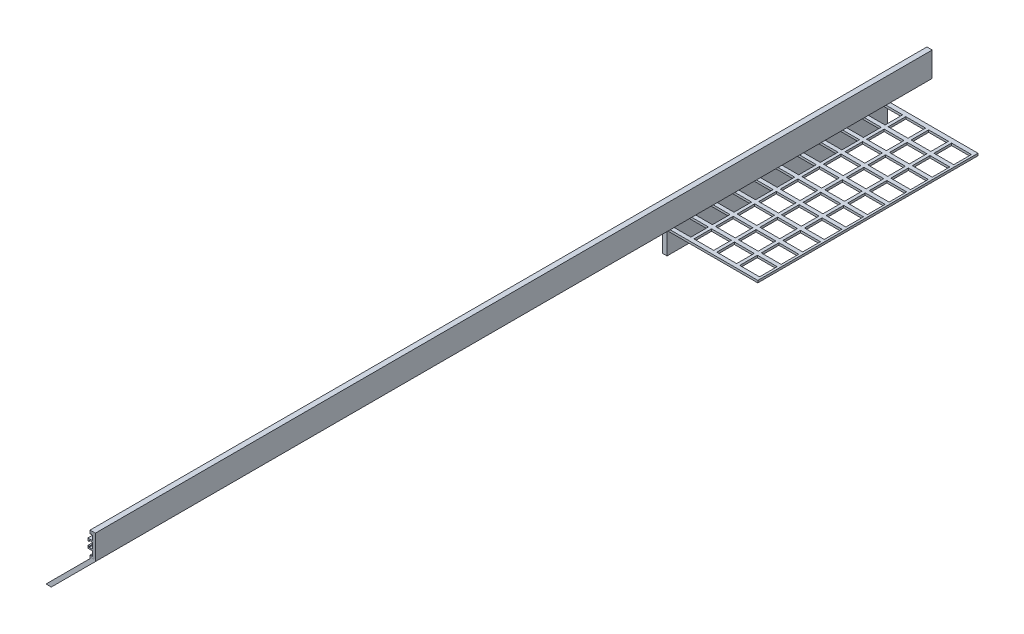
SolidWorks part; units mm, degrees
ref_plane "前视基准面" through (0, 0, 0) normal (0, 0, 1) x (1, 0, 0)
ref_plane "上视基准面" through (0, 0, 0) normal (0, 1, 0) x (1, 0, 0)
ref_plane "右视基准面" through (0, 0, 0) normal (1, 0, 0) x (0, 0, -1)
sketch "草图1" plane through (0, 0, 0) normal (0, 0, 1) x (1, 0, 0)
  line L0 (0, 0) -> (36.8328, 0) construction
  line L1 (3, -25) -> (3, 25)
  line L2 (3, 25) -> (-3, 25)
  line L3 (-3, 25) -> (-3, 21)
  line L4 (-3, 21) -> (0, 21)
  line L5 (0, 21) -> (0, 10)
  line L6 (0, 10) -> (-11, 10)
  line L7 (-11, 10) -> (-11, 4.6)
  line L8 (-11, 4.6) -> (-8, 4.6)
  line L9 (-8, 4.6) -> (-8, 7)
  line L10 (-8, 7) -> (0, 7)
  line L11 (0, 7) -> (0, -7)
  line L12 (-8, -7) -> (0, -7)
  line L13 (-8, -4.6) -> (-8, -7)
  line L14 (-11, -4.6) -> (-8, -4.6)
  line L15 (-11, -10) -> (-11, -4.6)
  line L16 (0, -10) -> (-11, -10)
  line L17 (0, -21) -> (0, -10)
  line L18 (-3, -21) -> (0, -21)
  line L19 (-3, -25) -> (-3, -21)
  line L20 (3, -25) -> (-3, -25)
  point P24 (3, 0)
  dimension "D1" = 25
  dimension "D2" = 6
  dimension "D3" = 3
  dimension "D4" = 4
  dimension "D5" = 3
  dimension "D6" = 10
  dimension "D7" = 4.6
  dimension "D8" = 8
  dimension "D9" = 3
extrude "凸台-拉伸1" add sketch "草图1" along normal mid plane 3000
sketch "草图2" plane through (0, 0, 0) normal (0, 0, 1) x (1, 0, 0)
  line L0 (3, -25) -> (3, 25) construction
  line L1 (3, 25) -> (-3, 25) construction
  line L2 (-3, 25) -> (-3, 21) construction
  line L3 (-3, -25) -> (3, -25) construction
  line L4 (-3, -21) -> (-3, -25) construction
  line L5 (3, -25) -> (3, 25)
  line L6 (3, 25) -> (-3, 25)
  line L7 (-3, 25) -> (-3, 21)
  line L8 (-3, -25) -> (3, -25)
  line L9 (-3, -21) -> (-3, -25)
  line L10 (-6, -21) -> (-6, -28)
  line L11 (-6, -28) -> (6, -28)
  line L12 (6, -28) -> (6, 28)
  line L13 (6, 28) -> (-6, 28)
  line L14 (-6, 28) -> (-6, 21)
  line L15 (-3, 21) -> (-6, 21)
  line L16 (-3, -21) -> (-6, -21)
  dimension "D1" = 3
extrude "凸台-拉伸2" add sketch "草图2" along normal mid plane 3000 separate body
sketch "草图3" plane through (0, 0, -1500) normal (0, 0, -1) x (-1, 0, 0)
  line L0 (6, -28) -> (106, -128)
  line L1 (6, -28) -> (-6, -28) construction
  line L2 (106, -128) -> (94, -128)
  line L3 (94, -128) -> (-6, -28)
  line L4 (6, -28) -> (-6, -28)
  dimension "D1" = 12
  dimension "D2" = 45
  dimension "D3" = 100
extrude "凸台-拉伸3" add sketch "草图3" against normal through all
sketch "草图4" plane through (0, 0, -1500) normal (0, 0, -1) x (-1, 0, 0)
  line L0 (94, -128) -> (106, -128) construction
  line L1 (106, -128) -> (-110, -128)
  line L3 (89.7158, -123) -> (-110, -123)
  line L4 (-110, -128) -> (-110, -123)
  line L5 (-6, -28) -> (-6, 28) construction
  line L6 (106, -128) -> (6, -28) construction
  line L7 (106, -128) -> (89.7158, -123)
  dimension "D1" = 104
  dimension "D2" = 5
extrude "凸台-拉伸4" add sketch "草图4" against normal blind 500
sketch "草图5" plane through (0, 0, -1500) normal (0, 0, -1) x (-1, 0, 0)
  line L0 (-110, -128) -> (106, -128) construction
  line L1 (106, -128) -> (96, -128)
  line L2 (106, -128) -> (106, -178)
  line L3 (106, -178) -> (96, -178)
  line L4 (96, -128) -> (96, -178)
  line L5 (106, -128) -> (6, -28) construction
  dimension "D1" = 10
  dimension "D2" = 50
extrude "凸台-拉伸5" add sketch "草图5" against normal blind 500
sketch "草图6" plane through (0, -128, 0) normal (0, -1, 0) x (1, 0, 0)
  line L0 (-96, -1000) -> (-96, -1500) construction
  line L1 (-96, -1490) -> (-51, -1490)
  line L2 (-96, -1490) -> (-96, -1450)
  line L3 (-96, -1450) -> (-51, -1450)
  line L4 (-51, -1490) -> (-51, -1450)
  line L5 (110, -1500) -> (-96, -1500) construction
  line L6 (-44, -1450) -> (1, -1450)
  line L7 (1, -1490) -> (1, -1450)
  line L8 (-44, -1490) -> (1, -1490)
  line L9 (-44, -1490) -> (-44, -1450)
  line L10 (8, -1450) -> (53, -1450)
  line L11 (53, -1490) -> (53, -1450)
  line L12 (8, -1490) -> (53, -1490)
  line L13 (8, -1490) -> (8, -1450)
  line L14 (60, -1450) -> (105, -1450)
  line L15 (105, -1490) -> (105, -1450)
  line L16 (60, -1490) -> (105, -1490)
  line L17 (60, -1490) -> (60, -1450)
  dimension "D1" = 10
  dimension "D2" = 40
  dimension "D3" = 45
  dimension "D4" = 4
extrude "切除-拉伸1" cut sketch "草图6" against normal up to surface up to face at (-59, -93, -333.3333)
pattern_linear "阵列(线性)1" count 10 spacing 49 along (0, 0, 1) of "切除-拉伸1"
sketch "草图7" plane through (0, 0, 1500) normal (0, 0, 1) x (1, 0, 0)
  line L0 (493.0939, -226) -> (-106.9061, -226) construction
  line L1 (65.5332, -226) -> (-163.3549, -226)
  line L2 (65.5332, -226) -> (65.5332, 57.3887)
  line L3 (65.5332, 57.3887) -> (-163.3549, 57.3887)
  line L4 (-163.3549, -226) -> (-163.3549, 57.3887)
extrude "切除-拉伸2" cut sketch "草图7" against normal blind 1100
